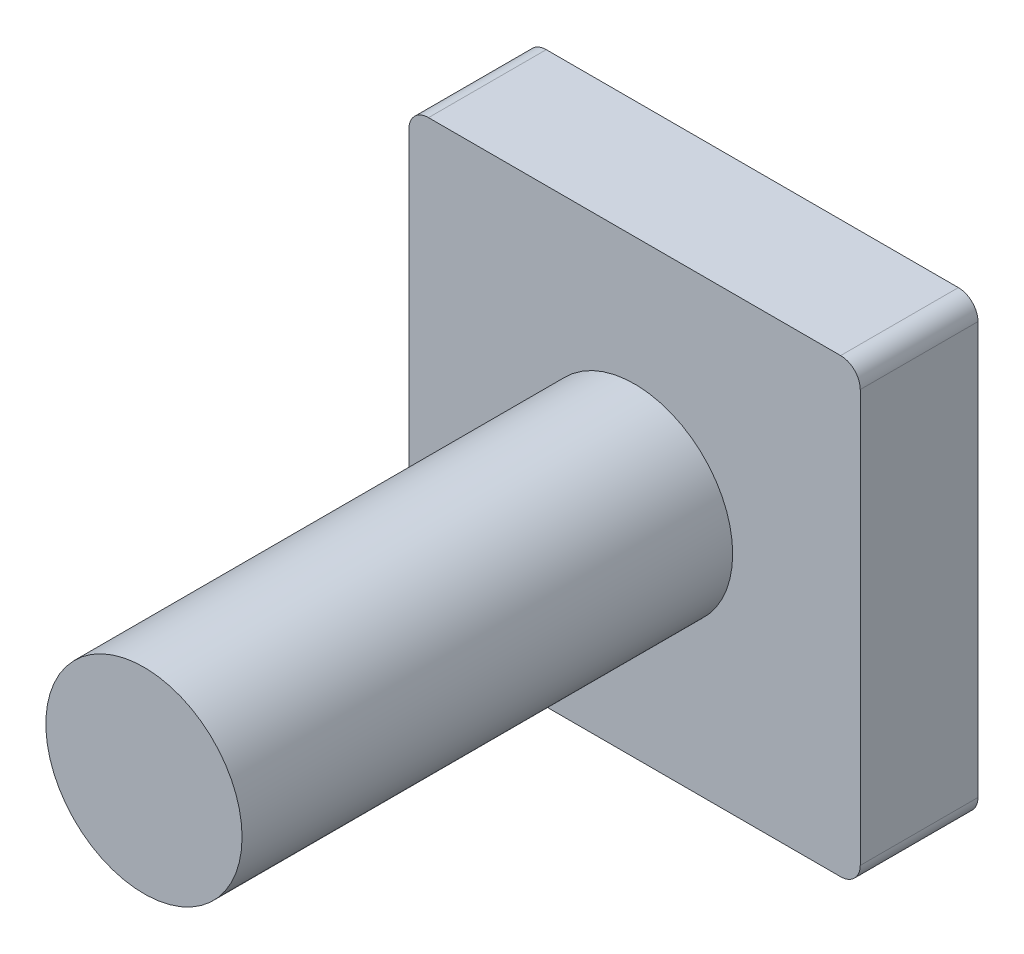
from build123d import *

# Parameters (mm, degrees)
SKETCH_1_R      = 5
EXTRUDE_1_DEPTH = 25
SKETCH_2_W      = 23
SKETCH_2_H      = 23
EXTRUDE_2_DEPTH = 6
FILLET_1_R      = 1


with BuildPart() as part:
    # 草图1 → 凸台-拉伸1 (new body)
    with BuildSketch(Plane.XY):
        Circle(SKETCH_1_R)
    extrude(amount=EXTRUDE_1_DEPTH)

    # 草图2 → 凸台-拉伸2 (add)
    with BuildSketch(Plane(origin=(0, 0, 0), x_dir=(-1, 0, 0), z_dir=(0, 0, -1))):
        Rectangle(SKETCH_2_W, SKETCH_2_H)
    extrude(amount=EXTRUDE_2_DEPTH)

    # 圆角1
    fillet_1_edges = [part.edges().sort_by_distance(p)[0] for p in [
        (11.5, 11.5, -3),
        (11.5, -11.5, -3),
        (-11.5, -11.5, -3),
        (-11.5, 11.5, -3),
    ]]
    fillet(fillet_1_edges, radius=FILLET_1_R)


solid = part.part
